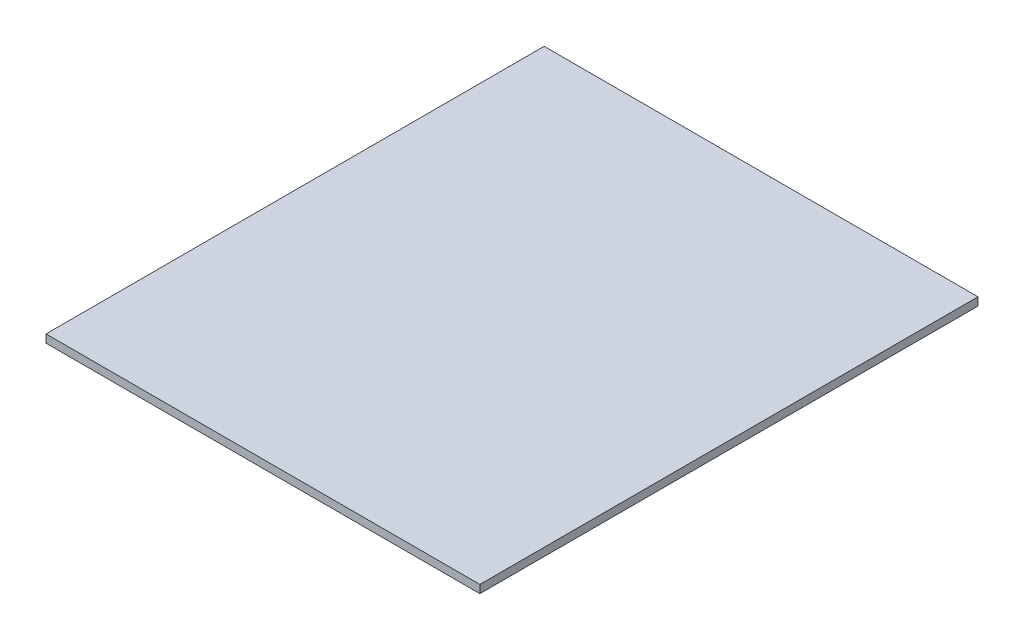
from build123d import *

# Parameters (mm, degrees)
SKETCH1_W           = 270
SKETCH1_H           = 310
BOSS_EXTRUDE1_DEPTH = 5


with BuildPart() as part:
    # Sketch1 → Boss-Extrude1 (new body)
    with BuildSketch(Plane(origin=(0, 0, 0), x_dir=(1, 0, 0), z_dir=(0, 1, 0))):
        Rectangle(SKETCH1_W, SKETCH1_H)
    extrude(amount=BOSS_EXTRUDE1_DEPTH)


solid = part.part
